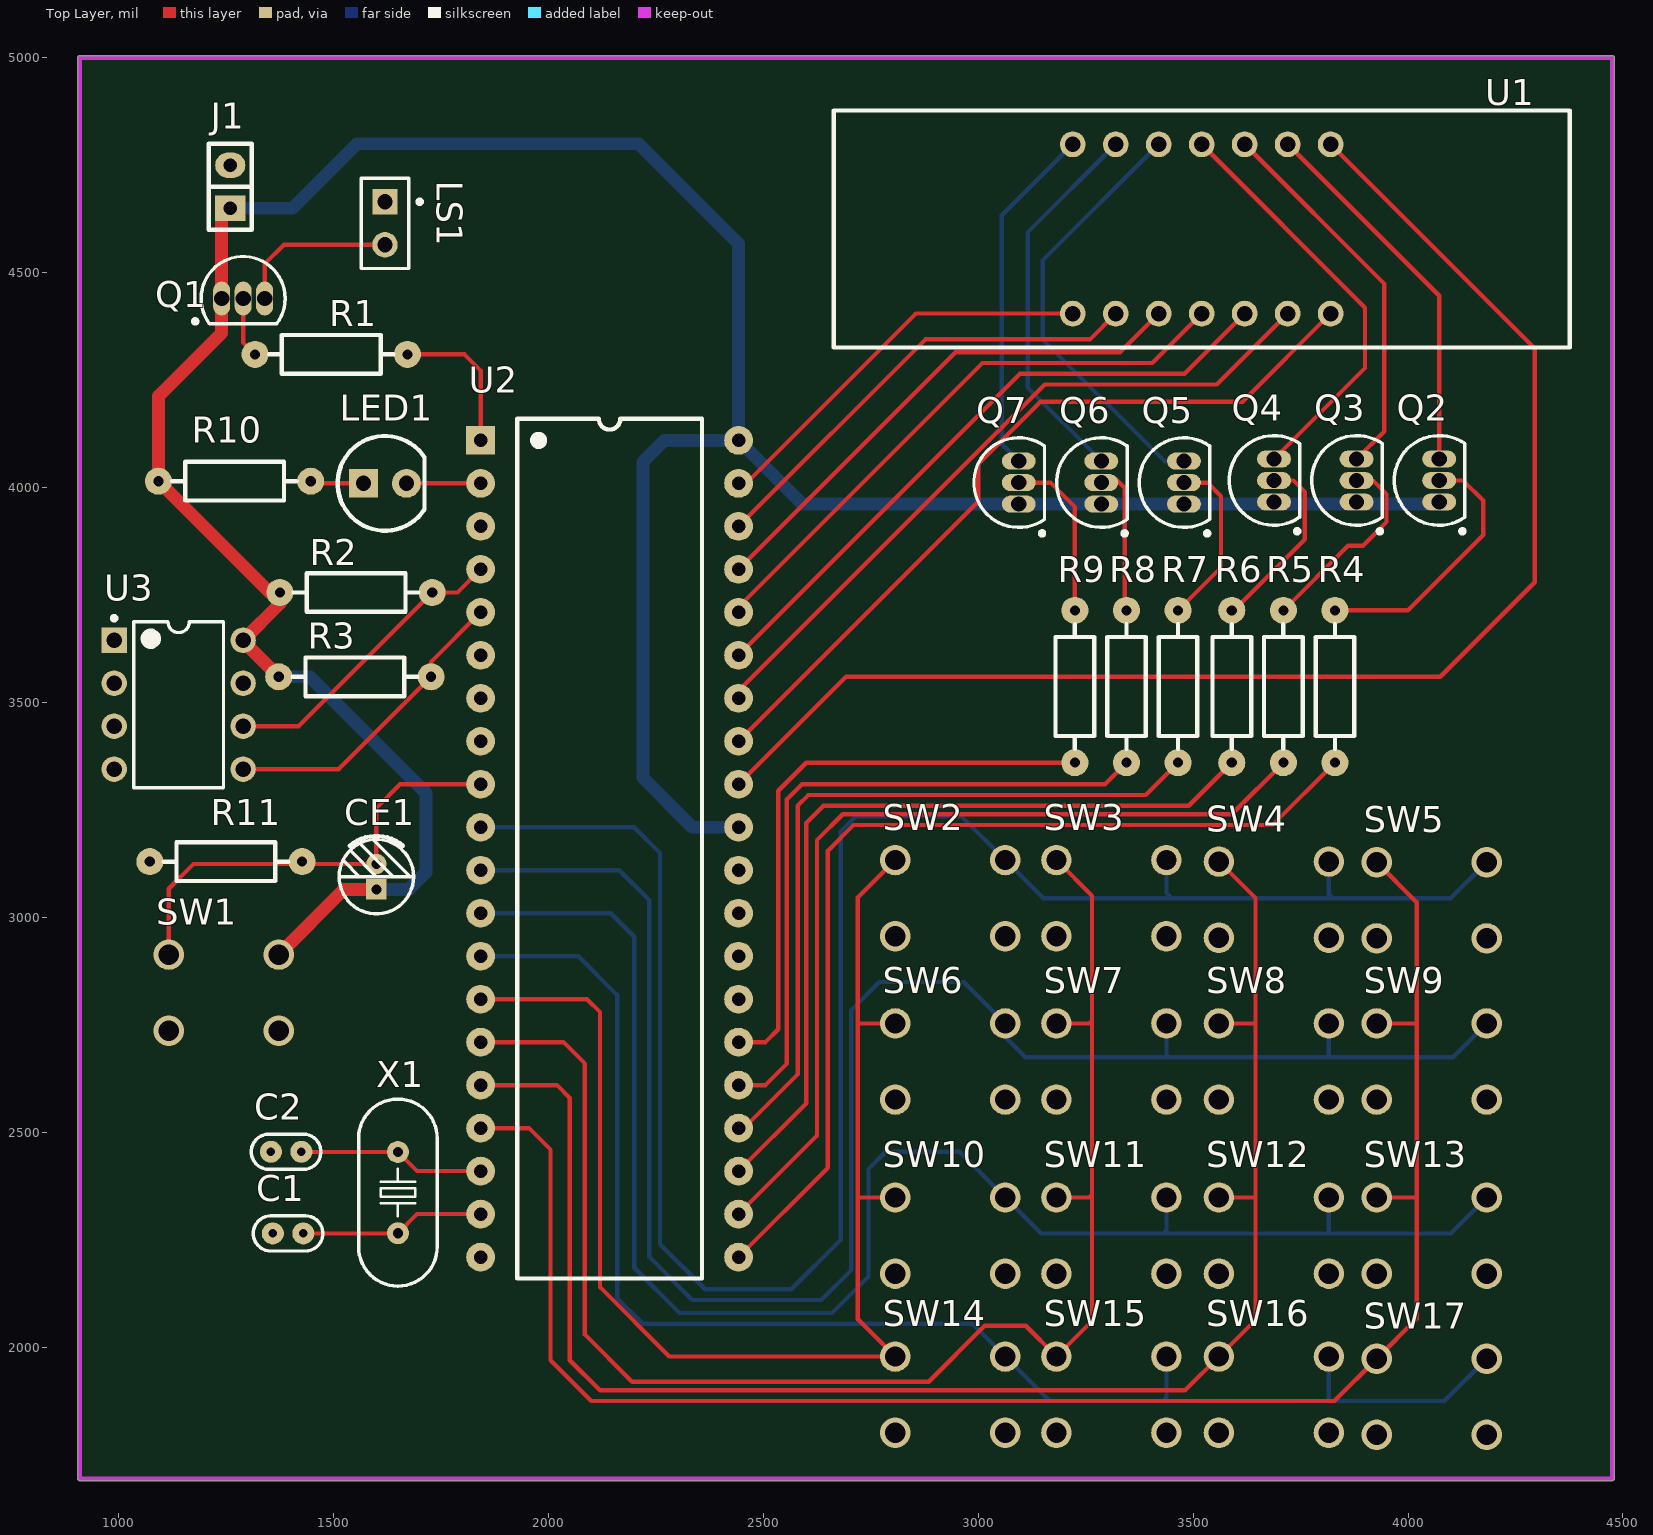
[diagram p0: Top Layer view]
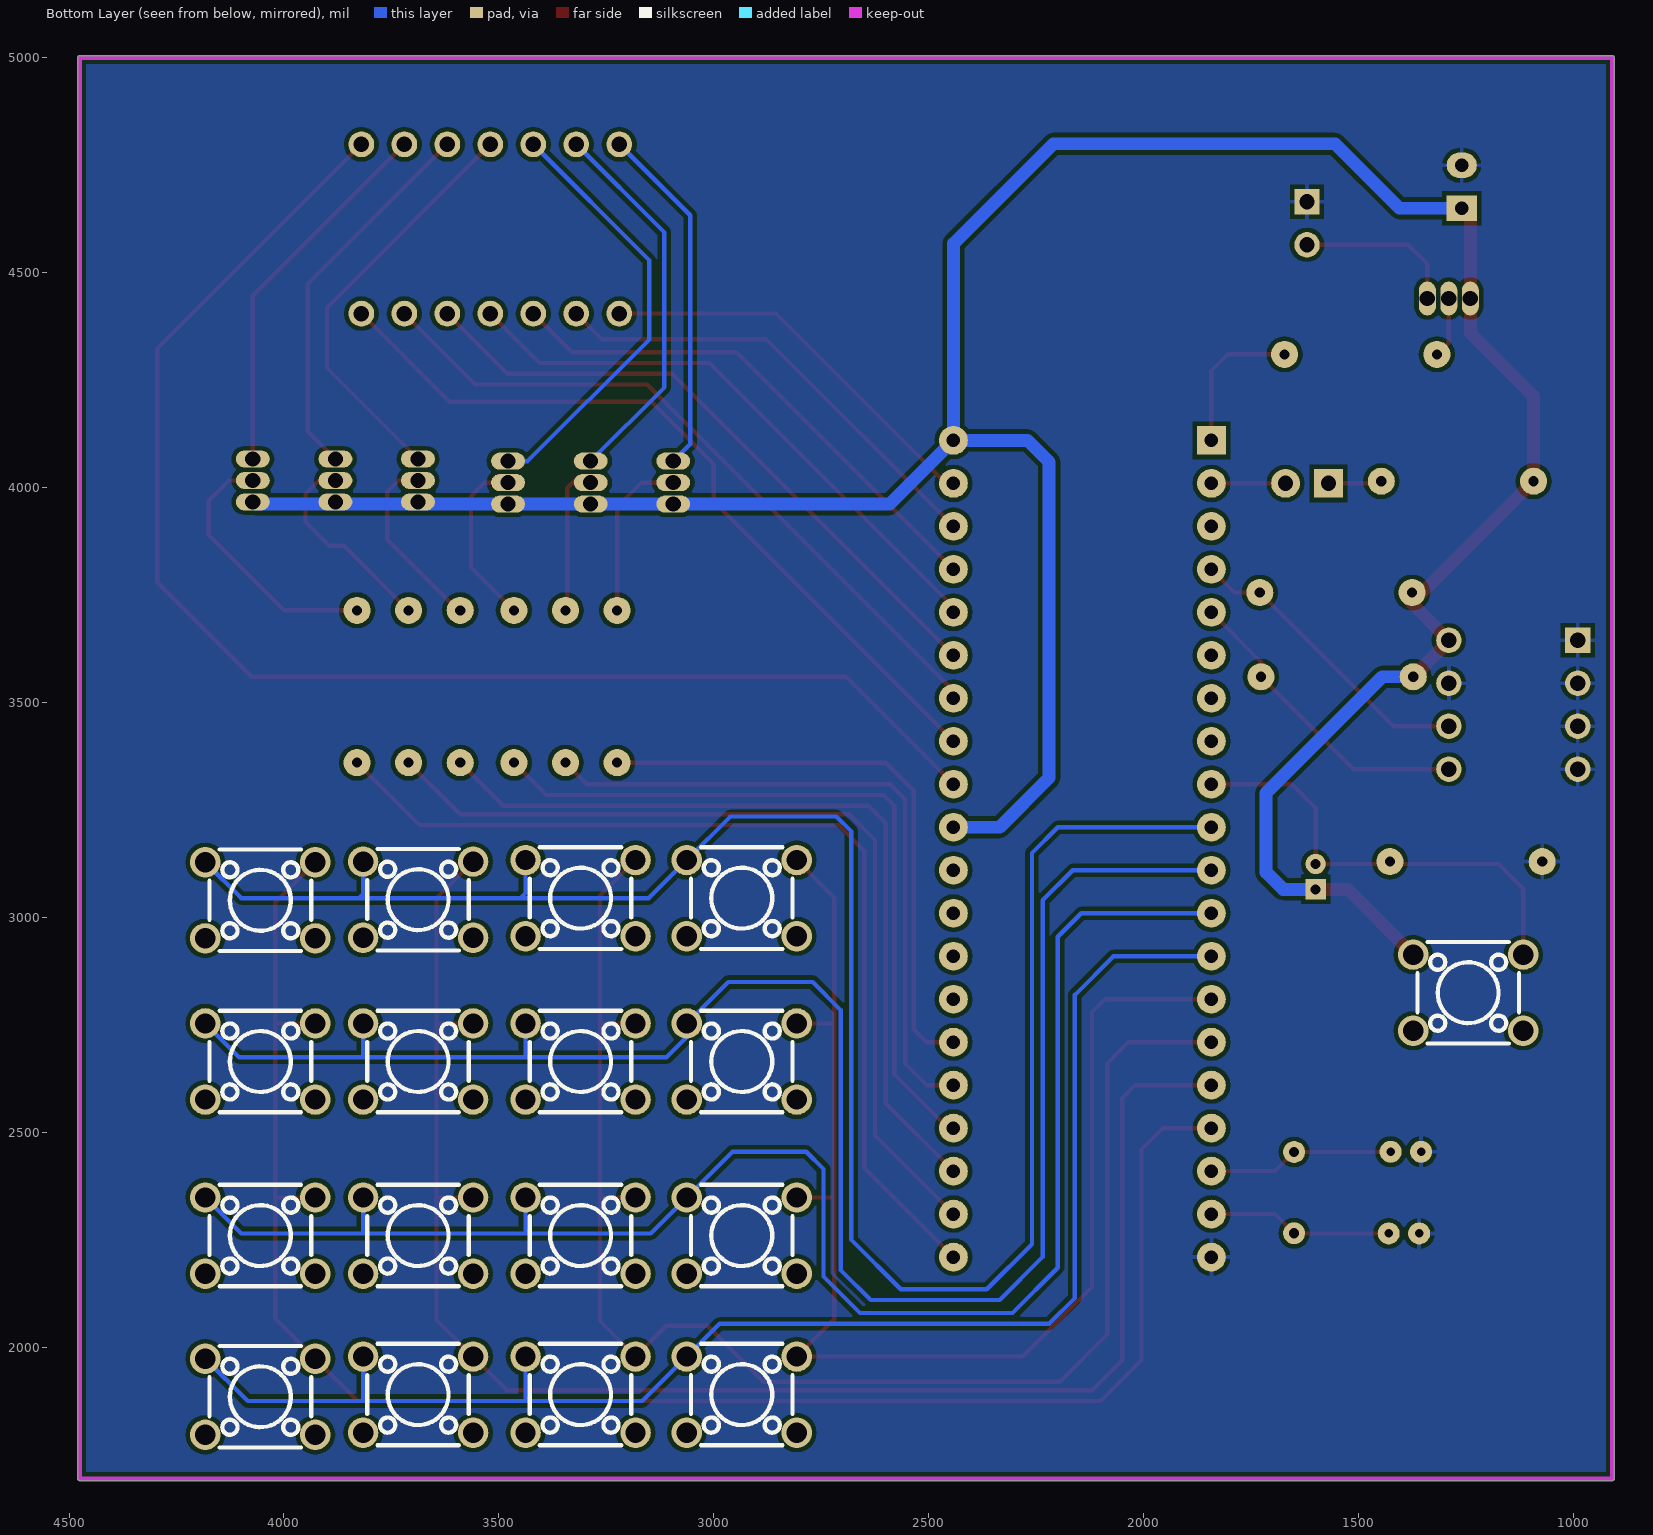
[diagram p1: Bottom Layer view, seen from below]
# Altium PCB MISC82700.PcbDoc
Units mil, origin at the board's own origin, x right, y up, seen from the top; angles counter-clockwise.
Board outline 3575.03 x 3315.03 mil, 2 copper layers (Top Layer, Bottom Layer); 45 components, 46 nets, 187 pads, 0 vias.

## Layer stack, top to bottom (the 12.6 mil dielectric is the usual default, probably not edited)
Top Solder: solder mask 0.4, Solder Resist, Dk 3.5
Top Layer: signal copper 1.4
Dielectric 1: dielectric 12.6, FR-4, Dk 4.8
Bottom Layer: signal copper 1.4
Bottom Solder: solder mask 0.4, Solder Resist, Dk 3.5

## Board outline
910,1689.98 cw(c910,1695) 904.99,1695 904.99,5000 cw(c910,5000) 910,5005.02 4475,5005.02 cw(c4475,5000) 4480.02,5000 4480.02,1695 cw(c4475,1695) 4475,1689.98

## Design rules (kind name [scope] priority, off if disabled: settings)
Clearance [All] p1: gap=10
MinimumSolderMaskSliver [All] p1: minsoldermaskwidth=0
PolygonConnect [All] p1: connectstyle=Relief reliefconductorwidth=10 reliefentries=4 polygonreliefangle="90 Angle" airgapwidth=10
RoutingVias [All] p1: holewidth=28 width=50 viastyle="Through Hole" minholewidth=28 minwidth=50 maxholewidth=28 maxwidth=50
SilkToSilkClearance [All] p1: silktosilkclearance=0
SilkToSolderMaskClearance [IsPad] p1: minsilkscreentomaskgap=0 clearancetoexposedcopper=TRUE
SolderMaskExpansion [All] p1: expansion=4
Width [All] p1: maxlimit=30 minlimit=10 preferedwidth=10
27 further rules are at their usual default settings.

## Components (designator, comment, footprint, x,y, rotation, side; value= is the part's Value field where it differs from the comment)
C1 "30PF" "CC 1.8*3.6" 1394.57,2265 r0 top
C2 "30PF" "CC 1.8*3.6" 1390,2455 r0 top
CE1 "47UF" "CAP 1.5*4*8" 1600,3095 r90 top
J1 "Female HDR1X2" Fe-HDR1X2/2.54-S 1260,4650 r90 top
LED1 "Red" "LED 5MM-B" 1620,4010 r0 top
LS1 "Bell" PIN2 1620,4665 r270 top
Q1 "PNP" TO-92A 1290,4440 r270 top
Q2 "NPN" TO-226-AA 4072.44,4016.73 r0 top
Q3 "NPN" TO-226-AA 3880.35,4016.73 r0 top
Q4 "NPN" TO-226-AA 3688.27,4016.73 r0 top
Q5 "NPN" TO-226-AA 3478.7,4011.73 r0 top
Q6 "NPN" TO-226-AA 3286.61,4011.73 r0 top
Q7 "NPN" TO-226-AA 3094.53,4011.73 r0 top
R1 "470" "RS 1/4W" 1495,4310 r180 top
R2 "10K" "RS 1/4W" 1552.66,3756.01 r180 top
R3 "10K" "RS 1/4W" 1550,3560 r180 top
R4 "1K" "RS 1/4W" 3830,3537.34 r90 top
R5 "1K" "RS 1/4W" 3710,3537.34 r90 top
R6 "1K" "RS 1/4W" 3590,3537.34 r90 top
R7 "1K" "RS 1/4W" 3465,3537.34 r90 top
R8 "1K" "RS 1/4W" 3345,3537.34 r90 top
R9 "1K" "RS 1/4W" 3225,3537.34 r90 top
R10 "100" "RS 1/4W" 1270,4015 r180 top
R11 "1K" "RS 1/4W" 1250,3130 r0 top
SW1 "3x6x5" 四脚轻触开关 1245,2825 r0 top
SW2 "3x6x5" 四脚轻触开关 2935,3045 r0 top
SW3 "3x6x5" 四脚轻触开关 3310,3045 r0 top
SW4 "3x6x5" 四脚轻触开关 3687.95,3041.42 r0 top
SW5 "3x6x5" 四脚轻触开关 4055,3040 r0 top
SW6 "3x6x5" 四脚轻触开关 2935,2665 r0 top
SW7 "3x6x5" 四脚轻触开关 3310,2665 r0 top
SW8 "3x6x5" 四脚轻触开关 3687.95,2665 r0 top
SW9 "3x6x5" 四脚轻触开关 4055,2665 r0 top
SW10 "3x6x5" 四脚轻触开关 2935,2260 r0 top
SW11 "3x6x5" 四脚轻触开关 3310,2260 r0 top
SW12 "3x6x5" 四脚轻触开关 3687.95,2260 r0 top
SW13 "3x6x5" 四脚轻触开关 4055,2260 r0 top
SW14 "3x6x5" 四脚轻触开关 2935,1890 r0 top
SW15 "3x6x5" 四脚轻触开关 3310,1890 r0 top
SW16 "3x6x5" 四脚轻触开关 3687.95,1890 r0 top
SW17 "3x6x5" 四脚轻触开关 4055,1885 r0 top
U1 "6-digit display_1" 6位数码管 3520,4601.85 r0 top
U2 "ATC89C52" DIP40 2142.46,3160 r0 top
U3 "24C02C" PDIP300-P8 1140,3495 r0 top
X1 "12MHz" "OSC HC-49S" 1650,2360 r270 top

## Footprints (in the part's own frame and the unit in brackets; to place one, negate y for a bottom-side part, rotate by r counter-clockwise, add the part's x,y. Pads: shape width x height; smd on the part's side, far side on the other; paste and mask are expansions set on the pad)
6位数码管 [mil]
  round 60 hole 36 paste+4 mask+4: 1(-300,-196.85) 2(-200,-196.85) 3(-100,-196.85) 4(0,-196.85) 5(100,-196.85) 6(200,-196.85) 7(300,-196.85) 8(300,196.85) 9(200,196.85) 10(100,196.85) 11(0,196.85) 12(-100,196.85) 13(-200,196.85) 14(-300,196.85)
  silkscreen extent -856,-276 856,276
"CAP 1.5*4*8" [mm] "脚距1.5mm直径4mm高度8mm"
  rect 1.2x1.2 hole 0.6: 1(-0.75,0)
  round 1.2 hole 0.6: 2(0.75,0)
  silkscreen extent -2.2,-2.2 2.41,2.2, body extent -2,-2 2.02,2, height 8.04
"CC 1.8*3.6" [mm] "脚距1.8mm直径3.6mm"
  round 1.3 hole 0.5: 1(-0.9,0) 2(0.9,0)
  silkscreen extent -2.05,-1.04 2.05,1.04, body extent -1.8,-0.8 1.8,0.8, height 3.6
DIP40 [mm]
  rect 1.7x1.7 hole 0.8: 1(-7.62,24.13)
  round 1.7 hole 0.8: 2(-7.62,21.59) 3(-7.62,19.05) 4(-7.62,16.51) 5(-7.62,13.97) 6(-7.62,11.43) 7(-7.62,8.89) 8(-7.62,6.35) 9(-7.62,3.81) 10(-7.62,1.27) 11(-7.62,-1.27) 12(-7.62,-3.81) 13(-7.62,-6.35) 14(-7.62,-8.89) 15(-7.62,-11.43) 16(-7.62,-13.97) 17(-7.62,-16.51) 18(-7.62,-19.05) 19(-7.62,-21.59) 20(-7.62,-24.13) 21(7.62,-24.13) 22(7.62,-21.59) 23(7.62,-19.05) 24(7.62,-16.51) 25(7.62,-13.97) 26(7.62,-11.43) 27(7.62,-8.89) 28(7.62,-6.35) 29(7.62,-3.81) 30(7.62,-1.27) 31(7.62,1.27) 32(7.62,3.81) 33(7.62,6.35) 34(7.62,8.89) 35(7.62,11.43) 36(7.62,13.97) 37(7.62,16.51) 38(7.62,19.05) 39(7.62,21.59) 40(7.62,24.13)
  silkscreen extent -5.46,-25.4 5.46,25.4, body extent -7.91,-26.19 7.65,26.16, height 4.7
Fe-HDR1X2/2.54-S [mil] "Connector; Header; 2x2 Position"
  rect 60x70 hole 32: 1(0,0)
  oval 60x70 hole 32: 2(100,0)
  silkscreen extent -50,-50 150,50, body extent -55,-48 155,50, height 335
"LED 5MM-B" [mm] "蓝色5mm直插LED"
  rect 1.7x1.7 hole 0.9: 1(-1.27,0)
  round 1.7 hole 0.9: 2(1.27,0)
  silkscreen extent -2.8,-2.8 2.33,2.8, body extent -2.85,-2.85 2.45,2.85, height 8.75
"OSC HC-49S" [mm]
  round 1.3 hole 0.6: 1(-2.4,0) 2(2.4,0)
  silkscreen extent -5.52,-2.32 5.52,2.33, body extent -5.52,-2.32 5.53,2.33, height 4.13
PDIP300-P8 [mm] "DIP, 8-Leads, Row Spacing 7.62mm, Pitch 2.54mm, Body 9.5x6.6mm"
  rect 1.5x1.5 hole 0.9: 1(-3.81,3.81)
  round 1.5 hole 0.9: 2(-3.81,1.27) 3(-3.81,-1.27) 4(-3.81,-3.81) 5(3.81,-3.81) 6(3.81,-1.27) 7(3.81,1.27) 8(3.81,3.81)
  silkscreen extent -3.93,-4.9 2.65,5.23, body extent -3.55,-4.9 3.55,4.9, height 5.34
PIN2 [mm] "Photosensitive Diode; 2 Leads"
  rect 1.5x1.5 hole 0.9: 1(0,0)
  round 1.5 hole 0.9: 2(2.54,0)
  silkscreen extent -1.4,-1.4 3.94,2.18
"RS 1/4W" [mm] "直插色环电阻，脚距9mm，直径2.3mm"
  round 1.6 hole 0.6: 1(-4.5,0) 2(4.5,0)
  silkscreen extent -3.68,-1.14 3.68,1.14, body extent -4.72,-1.16 4.73,1.16, height 2.32
TO-92A [mm] "TO, Flat Index; 3 In-Line, Axial Leads; Body Dia. 4.5mm; Leads 0.51 x 0.48 mm (max)"
  oval 2x1 hole 0.9: 1(0,-1.27) 2(0,0) 3(0,1.27)
  silkscreen extent -2.48,-2.95 1.5,2.48, body extent -2.48,-2.5 1.5,2.5, height 6.86
TO-226-AA [mm] "TO, Flat Index; 3 In-Line, Axial Leads; Body Dia. 4.8mm; Leads 0.55 x 0.51 mm (max)"
  oval 2x1 hole 0.9: 1(0,-1.27) 2(0,0) 3(0,1.27)
  silkscreen extent -2.65,-3.13 1.52,2.65, body extent -2.65,-2.66 1.52,2.66, height 5.33
四脚轻触开关 [mm]
  round 1.8 hole 1.2 paste+0 mask+0.102: 1(3.25,2.25) 2(-3.25,2.25) 3(3.25,-2.25) 4(-3.25,-2.25)

## Part data
C1 C2: library part CC, "Ceramic capacitor"
CE1: library part CE, "Through-hole electrolytic capacitor"
LED1: library part LED-5MM, "5mm through-hole LED"
LS1: "Electrical Bell"
Q1: library part 2N3906, "PNP General Purpose Amplifier"
Q2 Q3 Q4 Q5 Q6 Q7: "NPN Bipolar Transistor"
R1 R2 R3 R4 R5 R6 R7 R8 R9 R10 R11: library part R-S, "Color-band resistor"
SW1 SW2 SW3 SW4 SW5 SW6 SW7 SW8 SW9 SW10 SW11 SW12 SW13 SW14 SW15 SW16 SW17: library part "TSW 3x6", "3x6 tactile switch"
U1: library part 6位数码管_1
U2: library part STC89C52
U3: library part 24C02C-I/P, "2Kbit, 400kHz, 5V, I2C Serial EEPROM, 8-Pin PDIP, Industrial Temperature"
X1: library part XTAL-2P, "2-pin passive crystal"

## Nets (pads, with @x,y where several pads share a name; then routed paths per layer and width w, separated by ;. In a path a pad name is that pad's centre, name@x,y a point inside that pad or via, vN(x,y) a via of type N, cw(c..) or ccw(c..) an arc to the next point about the centre after c; other vN are vias at no path point)
GND: C1.1 C2.1 J1.2 LS1.1 R11.1 U2.20 U3.1 U3.2 U3.3 U3.4 U3.7
K0: SW2.1 SW3.1 SW4.1 SW5.1 U2.10 | length 4626.6
  Bottom Layer w10: U2.10 2200,3210 2260,3150 2260,2240 2365,2135 2565,2135 2680,2250 2680,3200 2715,3235 2961.54,3235 SW2.1 3151.54,3045 3450,3045 ; SW3.1 3437.95,3057.05 3450,3045 ; SW4.1 3815.91,3054.09 3825,3045 ; SW5.1 4099.37,3045 3825,3045 ; 3450,3045 3825,3045
K1: SW6.1 SW7.1 SW8.1 SW9.1 U2.11 | length 4184.1
  Bottom Layer w10: U2.11 2165,3110 2235,3040 2235,2210 2335,2110 2635,2110 2705,2180 2705,2785 2770,2850 2966.54,2850 SW6.1 3062.95,2722.05 3110,2675 3435,2675 ; SW7.1 3437.95,2677.95 3435,2675 ; SW8.1 3815.91,2675.91 3815,2675 ; SW9.1 4104.37,2675 3815,2675 ; 3435,2675 3815,2675
K2: SW10.1 SW11.1 SW12.1 SW13.1 U2.12 | length 3762.7
  Bottom Layer w10: U2.12 2145,3010 2200,2955 2200,2185 2305,2080 2660,2080 2745,2165 2745,2415 2785,2455 2956.54,2455 SW10.1 3146.54,2265 3430,2265 ; SW11.1 3437.95,2272.95 3430,2265 ; SW12.1 3815.91,2265.91 3815,2265 ; SW13.1 4099.37,2265 3815,2265 ; 3430,2265 3815,2265
K3: SW14.1 SW15.1 SW16.1 SW17.1 U2.13 | length 3433.8
  Bottom Layer w10: U2.13 2070,2910 2160,2820 2160,2115 2220,2055 2986.54,2055 SW14.1 3166.54,1875 3430,1875 ; SW15.1 3437.95,1882.95 3430,1875 ; SW16.1 3815.91,1875.91 3815,1875 ; SW17.1 4084.37,1875 3815,1875 ; 3430,1875 3815,1875
K4: SW2.2 SW6.2 SW10.2 SW14.2 U2.14 | length 3087.1
  Top Layer w10: U2.14 2090,2810 2120,2780 2120,2140 2281.42,1978.58 SW14.2 2720,2065.63 2720,2350 ; SW10.2 2721.42,2348.58 2720,2350 ; SW6.2 2723.58,2753.58 2720,2750 ; SW2.2 2720,3046.54 2720,2750 ; 2720,2350 2720,2750
K5: SW3.2 SW7.2 SW11.2 SW15.2 U2.15 | length 3514.2
  Top Layer w10: U2.15 2035,2710 2085,2660 2085,2030 2195,1920 2885,1920 3015,2050 3110.63,2050 SW15.2 3265,2061.54 3265,2355 ; SW11.2 3258.58,2348.58 3265,2355 ; SW7.2 3258.58,2753.58 3265,2760 ; SW3.2 3265,3050.63 3265,2760 ; 3265,2355 3265,2760
K6: SW4.2 SW8.2 SW12.2 SW16.2 U2.16 | length 3796.3
  Top Layer w10: U2.16 2020,2610 2050,2580 2050,1970 2120,1900 3481.42,1900 SW16.2 3645,2063.58 3645,2345 ; SW12.2 3641.42,2348.58 3645,2345 ; SW8.2 3641.42,2753.58 3645,2750 ; SW4.2 3645,3045 3645,2750 ; 3645,2345 3645,2750
K7: SW5.2 SW9.2 SW13.2 SW17.2 U2.17 | length 4095.5
  Top Layer w10: U2.17 1955,2510 2005,2460 2005,1970 2100,1875 3828.46,1875 SW17.2 4020,2066.54 4020,2350 ; SW13.2 4018.58,2348.58 4020,2350 ; SW9.2 4016.42,2753.58 4020,2750 ; SW5.2 4020,3035.63 4020,2750 ; 4020,2350 4020,2750
NetC1_2: C1.2 U2.19 X1.2 | length 431.1
  Top Layer w10: C1.2 1649.49,2265 X1.2 1694.49,2310 U2.19
NetC2_2: C2.2 U2.18 X1.1 | length 435.7
  Top Layer w10: C2.2 1425.94,2454.49 X1.1 1694.49,2410 U2.18
NetCE1_2: CE1.2 R11.2 SW1.2 U2.9 | length 1055.9
  Top Layer w10: SW1.2 1117.05,3067.05 1174.53,3124.53 CE1.2 1600,3255 1655,3310 U2.9
NetLED1_1: LED1.1 R10.1 | length 124.9
  Top Layer w10: R10.1 1452.17,4010 LED1.1
NetLED1_2: LED1.2 U2.2 | length 172.5
  Top Layer w10: LED1.2 U2.2
NetLS1_2: LS1.2 Q1.3 | length 378.6
  Top Layer w10: Q1.3 1340,4520 1385,4565 LS1.2
NetQ1_2: Q1.2 R1.2 | length 141.5
  Top Layer w10: Q1.2 1290,4337.83 R1.2
NetQ2_2: Q2.2 R4.2 | length 619.6
  Top Layer w10: R4.2 3999.5,3714.5 4175,3890 4175,3970 4128.27,4016.73 Q2.2
NetQ2_3: Q2.3 U1.9 | length 878
  Top Layer w10: U1.9 4072.44,4446.26 Q2.3
NetQ3_2: Q3.2 R5.2 | length 472.9
  Top Layer w10: R5.2 3860.5,3865 3895,3865 3950,3920 3950,3985 3918.27,4016.73 Q3.2
NetQ3_3: Q3.3 U1.10 | length 893.4
  Top Layer w10: U1.10 3945,4473.7 3945,4131.38 Q3.3
NetQ4_2: Q4.2 R6.2 | length 431.4
  Top Layer w10: R6.2 3594.5,3714.5 3760,3880 3760,3990 3733.27,4016.73 Q4.2
NetQ4_3: Q4.3 U1.11 | length 977.1
  Top Layer w10: U1.11 3900,4418.7 3900,4278.46 Q4.3
NetQ5_2: Q5.2 R7.2 | length 406.4
  Top Layer w10: R7.2 3565,3814.5 3565,3980 3533.27,4011.73 Q5.2
NetQ5_3: Q5.3 U1.12 | length 1011.6
  Bottom Layer w10: U1.12 3150,4528.7 3150,4345 3433.27,4061.73 Q5.3
NetQ6_2: Q6.2 R8.2 | length 352.7
  Top Layer w10: Q6.2 3294.88,4020 3320,4020 3340.98,3999.02 3340.98,3718.52 R8.2
NetQ6_3: Q6.3 U1.13 | length 893
  Bottom Layer w10: Q6.3 3115,4233.35 3115,4593.7 U1.13
NetQ7_2: Q7.2 R9.2 | length 394.5
  Top Layer w10: Q7.2 3168.27,4011.73 3225,3955 R9.2
NetQ7_3: Q7.3 U1.14 | length 821.7
  Bottom Layer w10: Q7.3 3055,4101.26 3055,4633.7 U1.14
NetR1_1: R1.1 U2.1 | length 348.4
  Top Layer w10: R1.1 1805,4310 1842.46,4272.54 U2.1
NetR2_1: R2.1 U2.4 U3.6 | length 703.7
  Top Layer w10: U3.6 1418.82,3445 R2.1 1788.47,3756.01 U2.4
NetR3_1: R3.1 U2.5 U3.5 | length 724
  Top Layer w10: U3.5 1512.17,3345 R3.1 1727.17,3594.7 U2.5
NetR4_1: R4.1 U2.21 | length 2295.9
  Top Layer w10: U2.21 2650,2417.54 2650,3155 2710,3215 3684.83,3215 R4.1
NetR5_1: R5.1 U2.22 | length 2105.2
  Top Layer w10: U2.22 2625,2492.54 2625,3180 2685,3240 3589.83,3240 R5.1
NetR6_1: R6.1 U2.23 | length 1923.3
  Top Layer w10: U2.23 2600,2567.54 2600,3220 2640,3260 3489.83,3260 R6.1
NetR7_1: R7.1 U2.24 | length 1740.8
  Top Layer w10: U2.24 2455,2510 2580,2635 2580,3260 2605,3285 3389.83,3285 R7.1
NetR8_1: R8.1 U2.25 | length 1573.5
  Top Layer w10: U2.25 2505,2610 2555,2660 2555,3275 2590,3310 3294.83,3310 R8.1
NetR9_1: R9.1 U2.26 | length 1377
  Top Layer w10: U2.26 2505,2710 2535,2740 2535,3295 2600.17,3360.17 R9.1
NetU1_1: U1.1 U2.39 | length 941.1
  Top Layer w10: U2.39 2460,4010 2855,4405 U1.1
NetU1_2: U1.2 U2.38 | length 1082.6
  Top Layer w10: U2.38 2877.46,4345 3260,4345 U1.2
NetU1_3: U1.3 U2.37 | length 1224
  Top Layer w10: U2.37 2947.46,4315 3330,4315 U1.3
NetU1_4: U1.4 U2.36 | length 1372.7
  Top Layer w10: U2.36 2442.46,3722.46 3010,4290 3405,4290 U1.4
NetU1_5: U1.5 U2.35 | length 1506.8
  Top Layer w10: U2.35 3097.46,4265 3480,4265 U1.5
NetU1_6: U1.6 U2.34 | length 1658.5
  Top Layer w10: U2.34 2442.46,3527.46 3155,4240 3555,4240 U1.6
NetU1_7: U1.7 U2.33 | length 1840.9
  Top Layer w10: U2.33 3000,3967.54 3000,4055 3145,4200 3615,4200 U1.7
NetU1_8: U1.8 U2.32 | length 3262.7
  Top Layer w10: U2.32 2692.46,3560 4075,3560 4295,3780 4295,4323.7 U1.8
VCC: CE1.1 J1.1 Q1.1 Q2.1 Q3.1 Q4.1 Q5.1 Q6.1 Q7.1 R2.2 R3.2 R10.2 SW1.1 U2.31 U2.40 U3.8 | length 7160.4
  Top Layer w30: J1.1 1240,4630 Q1.1 1240,4360 1092.83,4212.83 R10.2 1351.83,3756.01 R2.2 1375.5,3730.5 U3.8 1290,3642.83 R3.2 ; SW1.1 1524.84,3065.47 CE1.1
  Bottom Layer w30: J1.1 1405,4650 1555,4800 2210,4800 2442.46,4567.54 U2.40 ; R3.2 1445,3560 1715,3290 1715,3105 1675.47,3065.47 CE1.1 ; U2.31 2335,3210 2220,3325 2220,4060 2270,4110 U2.40 ; Q2.1 4067.44,3961.73 3880.35,3961.73 Q5.1 Q6.1 Q7.1 2590.73,3961.73 U2.40
pads on no net: SW1.3 SW1.4 SW2.3 SW2.4 SW3.3 SW3.4 SW4.3 SW4.4 SW5.3 SW5.4 SW6.3 SW6.4 SW7.3 SW7.4 SW8.3 SW8.4 SW9.3 SW9.4 SW10.3 SW10.4 SW11.3 SW11.4 SW12.3 SW12.4 SW13.3 SW13.4 SW14.3 SW14.4 SW15.3 SW15.4 SW16.3 SW16.4 SW17.3 SW17.4 U2.3 U2.6 U2.7 U2.8 U2.27 U2.28 U2.29 U2.30

## Polygon pours and split planes (outlines as drawn)
GND on Bottom Layer "D" (solid, remove dead copper, pour order 0): 360,5145 400,5185 4625,5185 4625,1630 4515,1520 4465,1570 625,1570

## Keep-outs
Keep-Out Layer:
  lines w10: 1000,5000 4475,5000 4475,1695 1000,1695 910,1695 910,3675 910,5000 1035,5000